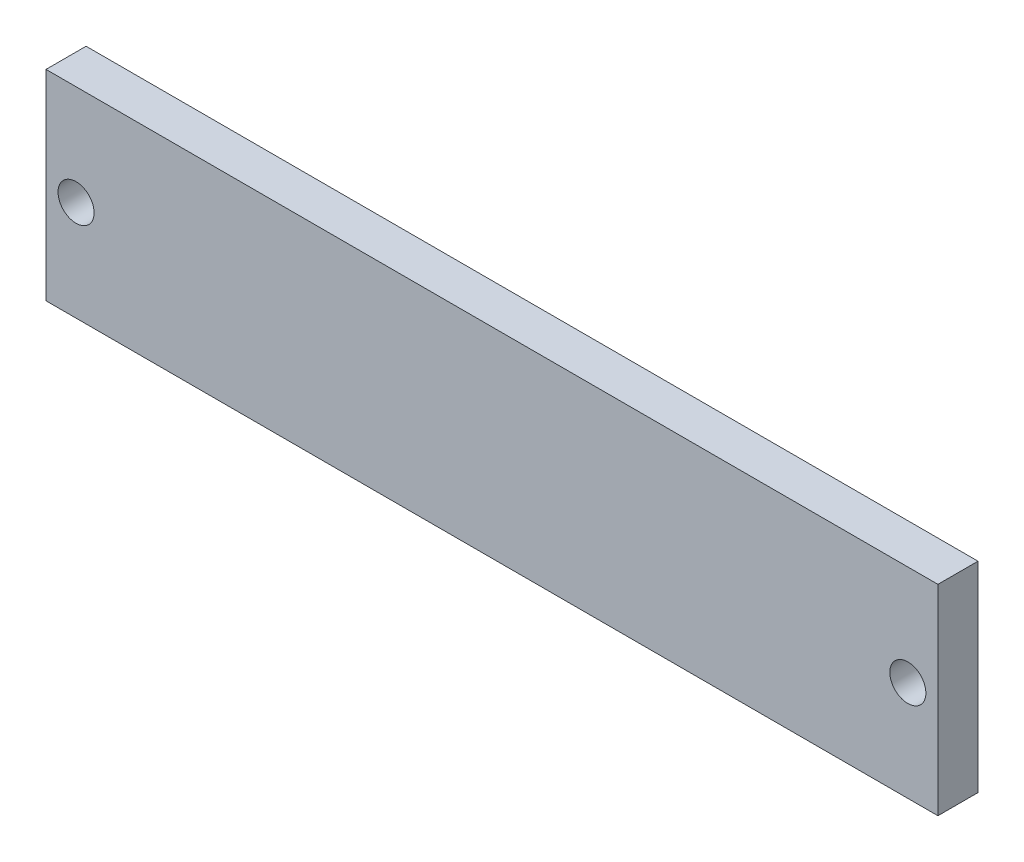
from build123d import *

# Parameters (mm, degrees)
SKETCH1_W           = 445
SKETCH1_H           = 100
SKETCH1_R           = 9
BOSS_EXTRUDE1_DEPTH = 20


with BuildPart() as part:
    # Sketch1 → Boss-Extrude1 (new body)
    with BuildSketch(Plane.XY):
        with Locations((222.5, 50)):
            Rectangle(SKETCH1_W, SKETCH1_H)
        with Locations((15, 50)):
            Circle(SKETCH1_R, mode=Mode.SUBTRACT)
        with Locations(Location((430, 50, 0), (0, 0, 180))):
            Circle(SKETCH1_R, mode=Mode.SUBTRACT)
    extrude(amount=BOSS_EXTRUDE1_DEPTH)


solid = part.part
